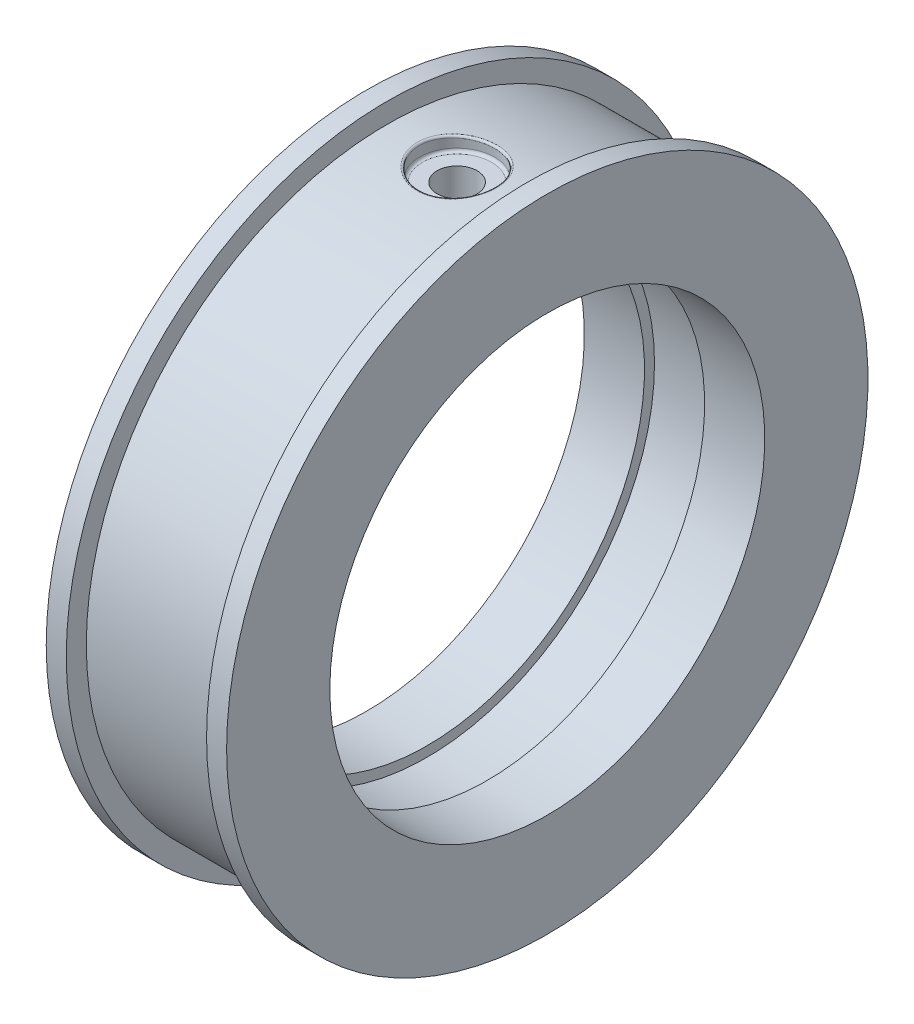
SolidWorks part; units mm, degrees
ref_plane "Front Plane" through (0, 0, 0) normal (0, 0, 1) x (1, 0, 0)
ref_plane "Top Plane" through (0, 0, 0) normal (0, 1, 0) x (1, 0, 0)
ref_plane "Right Plane" through (0, 0, 0) normal (1, 0, 0) x (0, 0, -1)
sketch "Sketch1" plane through (0, 0, 0) normal (0, 0, 1) x (1, 0, 0)
  line L0 (-19.0368, 0) -> (19.2228, 0) construction
  line L1 (-8.3897, 21.7) -> (-8.3897, 32)
  line L2 (-8.3897, 32) -> (-6.3897, 32)
  line L3 (-6.3897, 32) -> (-6.3897, 30)
  line L4 (-6.3897, 30) -> (7.6103, 30)
  line L5 (7.6103, 30) -> (7.6103, 32)
  line L6 (7.6103, 32) -> (9.6103, 32)
  line L7 (9.6103, 32) -> (9.6103, 21.7)
  line L8 (9.6103, 21.7) -> (3.6103, 21.7)
  line L9 (3.6103, 21.7) -> (3.6103, 22.7)
  line L10 (3.6103, 22.7) -> (-2.3897, 22.7)
  line L11 (-2.3897, 22.7) -> (-2.3897, 21.7)
  line L12 (-2.3897, 21.7) -> (-8.3897, 21.7)
  dimension "D2" = 18
  dimension "D3" = 14
  dimension "D4" = 2
  dimension "D5" = 21.7
  dimension "D6" = 21.7
  dimension "D7" = 22.7
  dimension "D8" = 6
  dimension "D9" = 6
  dimension "D10" = 30
  dimension "D11" = 32
  dimension "D12" = 32
revolve "Revolve1" add sketch "Sketch1" angle 360 about L0
ref_plane "Plane1" through (0, 30, 0) normal (0, 1, 0) x (1, 0, 0)
sketch "Sketch2" plane through (0, 30, 0) normal (0, 1, 0) x (1, 0, 0)
  line L0 (-6.3897, 0) -> (7.6103, 0)
  line L1 (-6.3897, -32) -> (-6.3897, 32) construction
  line L2 (7.6103, 30) -> (7.6103, -30) construction
hole_wizard "Hole1" positions "Sketch3" profile "Sketch4" legacy
sketch "Sketch3" plane through (0, 30, 0) normal (0, 1, 0) x (1, 0, 0)
  line L0 (-6.3897, 0) -> (7.6103, 0) construction
  point P0 (0.6103, 0)
sketch "Sketch4" plane through (0.6103, 30, 0) normal (1, 0, 0) x (0, 0, 1)
  line L0 (0, 0) -> (0, 1.5)
  line L1 (0, 1.5) -> (3.75, 1.5)
  line L2 (3.75, 1.5) -> (3.75, 0)
  line L3 (3.75, 0) -> (0, 0)
  line L4 (0, 110) -> (0, -10) construction
  dimension "直径" = 7.5
  dimension "深度" = 1.5
hole_wizard "Hole2" positions "Sketch5" profile "Sketch6" legacy
sketch "Sketch5" plane through (0, 28.5, 0) normal (0, 1, 0) x (1, 0, 0)
  point P0 (0.6103, 0)
sketch "Sketch6" plane through (0.6103, 28.5, 0) normal (1, 0, 0) x (0, 0, 1)
  line L0 (0, 0) -> (0, 5.8)
  line L1 (0, 5.8) -> (2, 5.8)
  line L2 (2, 5.8) -> (2, 0)
  line L3 (2, 0) -> (0, 0)
  line L4 (0, 110) -> (0, -10) construction
  dimension "直径" = 4
  dimension "深度" = 5.8
ref_plane "Plane2" through (0, -30, 0) normal (0, -1, 0) x (-1, 0, 0)
sketch "Sketch8" plane through (0, -30, 0) normal (0, -1, 0) x (-1, 0, 0)
  line L0 (6.3897, 0) -> (-7.6103, 0) construction
  line L1 (6.3897, 0) -> (-7.6103, 0)
hole_wizard "Dowel Hole1" positions "Sketch9" profile "Sketch10" hole size "Ø4.0" standard "GB"
sketch "Sketch9" plane through (0, -30, 0) normal (0, -1, 0) x (-1, 0, 0)
  line L0 (6.3897, 0) -> (-7.6103, 0) construction
  point P0 (-0.6103, 0)
sketch "Sketch10" plane through (0.6103, -30, 0) normal (1, 0, 0) x (0, 0, -1)
  line L0 (0, 0) -> (0, 5.2017)
  line L1 (0, 5.2017) -> (2, 4)
  line L2 (2, 4) -> (2, 0)
  line L5 (2, 0) -> (0, 0)
  line L10 (0, 5.2017) -> (-2, 4) construction
  line L11 (0, -6.35) -> (0, 107.95) construction
  dimension "孔直径" = 4
  dimension "孔深度" = 4
  dimension "导头角度" = 118
fillet "Fillet1" radius 0.2 1 edges at (1.44, 29.7763, -3.6571)
fillet "Fillet2" radius 0.3 1 edges at (0.6103, 28.5, 3.75)
